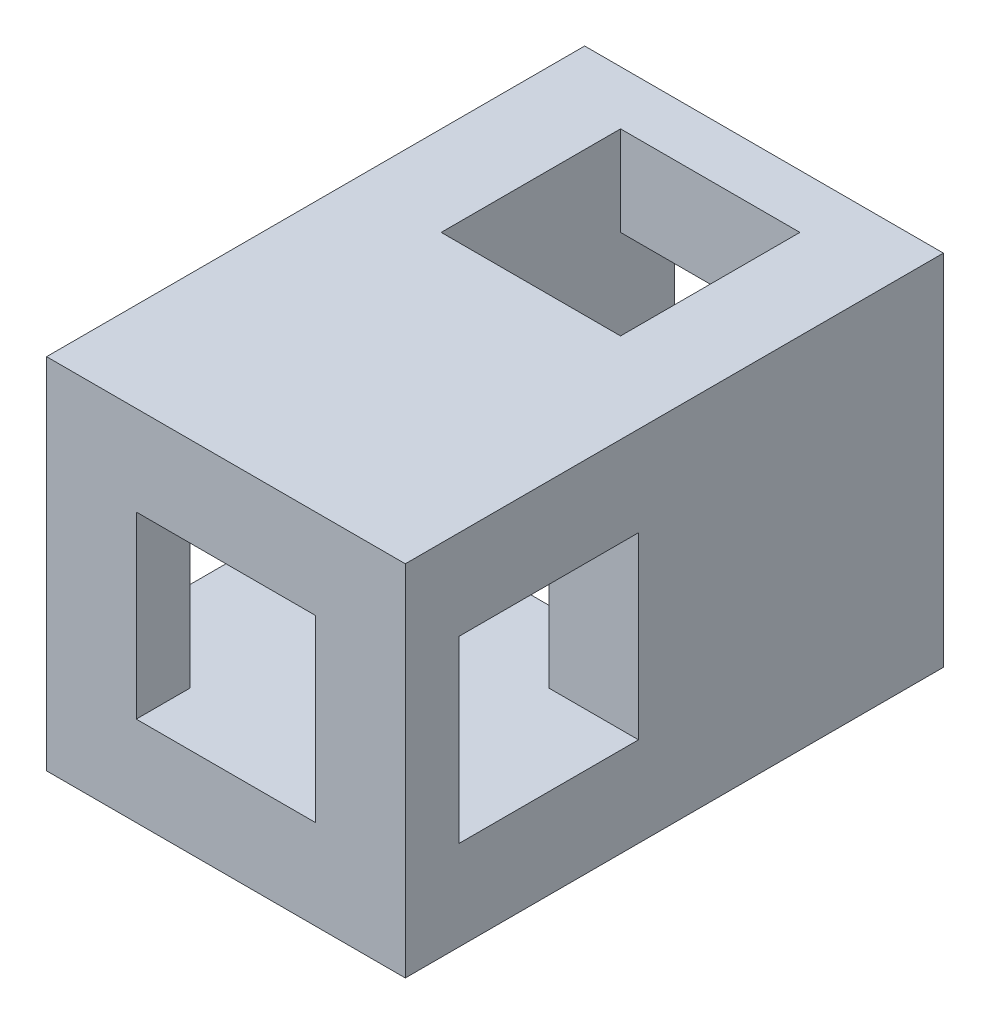
from build123d import *

# Parameters (mm, degrees)
SKETCH1_W           = 10
SKETCH1_H           = 10
SKETCH1_W_2         = 5
SKETCH1_H_2         = 5
BOSS_EXTRUDE1_DEPTH = 15
SKETCH2_W           = 5
SKETCH2_H           = 5
CUT_EXTRUDE1_DEPTH  = 19.708286934
SKETCH3_W           = 5
SKETCH3_H           = 5
CUT_EXTRUDE2_DEPTH  = 19.708286934


with BuildPart() as part:
    # Sketch1 → Boss-Extrude1 (new body)
    with BuildSketch(Plane.XY):
        Rectangle(SKETCH1_W, SKETCH1_H)
        Rectangle(SKETCH1_W_2, SKETCH1_H_2, mode=Mode.SUBTRACT)
    extrude(amount=BOSS_EXTRUDE1_DEPTH)

    # Sketch2 → Cut-Extrude1 (cut, through all)
    with BuildSketch(Plane(origin=(0, 5, 0), x_dir=(1, 0, 0), z_dir=(0, 1, 0))):
        with Locations((0, -4)):
            Rectangle(SKETCH2_W, SKETCH2_H)
    extrude(amount=-CUT_EXTRUDE1_DEPTH, mode=Mode.SUBTRACT)

    # Sketch3 → Cut-Extrude2 (cut, through all)
    with BuildSketch(Plane(origin=(5, 0, 0), x_dir=(0, 0, -1), z_dir=(1, 0, 0))):
        with Locations((-11, 0)):
            Rectangle(SKETCH3_W, SKETCH3_H)
    extrude(amount=-CUT_EXTRUDE2_DEPTH, mode=Mode.SUBTRACT)


solid = part.part
